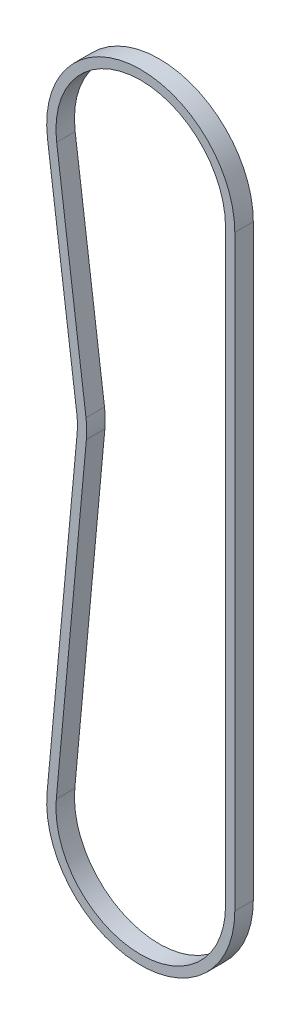
SolidWorks part; units mm, degrees
ref_plane "前视基准面" through (0, 0, 0) normal (0, 0, 1) x (1, 0, 0)
ref_plane "上视基准面" through (0, 0, 0) normal (0, 1, 0) x (1, 0, 0)
ref_plane "右视基准面" through (0, 0, 0) normal (1, 0, 0) x (0, 0, -1)
sketch "草图2" plane through (0, 0, 0) normal (0, 0, 1) x (1, 0, 0)
  line L0 (0, 0) -> (1, 0) construction
  line L1 (0, 0) -> (0, 1) construction
  line L2 (-90.8481, -11.9063) -> (-59.1519, -253.7557)
  line L3 (-58.7614, -274.0676) -> (-91.2386, -626.5945)
  line L4 (91.625, -635) -> (91.625, 0)
  arc A0 (91.625, 0) -> (-90.8481, -11.9063) centre (0, 0) ccw
  arc A1 (-59.1519, -253.7557) -> (-58.7614, -274.0676) centre (-150, -265.6621) cw
  arc A2 (-91.2386, -626.5945) -> (91.625, -635) centre (0, -635) ccw
extrude "拉伸-薄壁1" add sketch "草图2" along normal mid plane 20 thin
